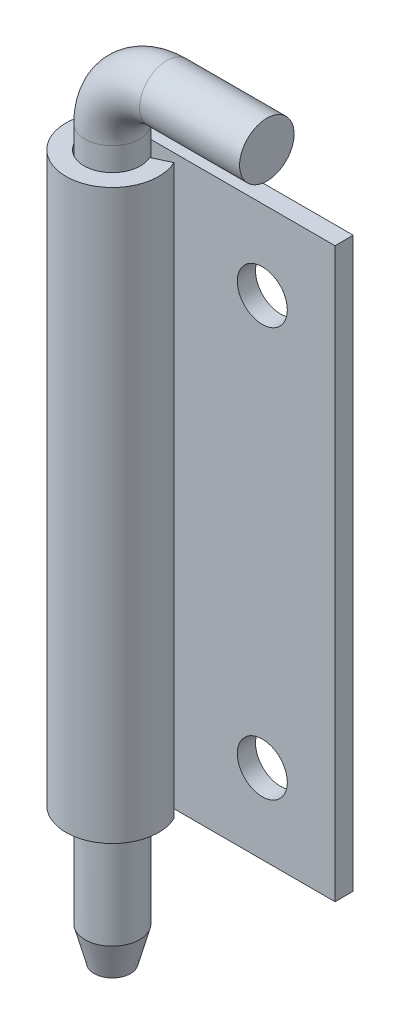
from build123d import *

# Parameters (mm, degrees)
SKETCH_2_R          = 3
EXTRUDE_1_DEPTH     = 62.5
SKETCH_5_R          = 2.75
CUT_EXTRUDE_2_DEPTH = 92.903210052
CHAMFER_1_SIZE      = 1
CHAMFER_1_SIZE2     = 3.732050808


with BuildPart() as part:
    # 扫描1: sweep along a path in 草图1
    with BuildLine(Plane.XY) as sweep_1_path:
        Line((0, 0), (0, 80))
        ThreePointArc((0, 80), (1.757359313, 84.242640687), (6, 86))
        Line((6, 86), (17, 86))
    # 草图2 → 扫描1 (sweep)
    with BuildSketch(Plane(origin=(0, 0, 0), x_dir=(1, 0, 0), z_dir=(0, 1, 0))):
        Circle(SKETCH_2_R)
    sweep(path=sweep_1_path.line)

    # 倒角1
    chamfer_1_edges = [part.edges().sort_by_distance(p)[0] for p in [
        (-3, 0, 0),
    ]]
    chamfer_1_side = [part.faces().sort_by_distance(p)[0] for p in [
        (0, 0, 0),
    ]]
    chamfer(chamfer_1_edges, length=CHAMFER_1_SIZE, length2=CHAMFER_1_SIZE2, reference=chamfer_1_side[0])


with BuildPart() as body_2:
    # 草图3 → 凸台-拉伸1 (new body)
    with BuildSketch(Plane(origin=(0, 15, 0), x_dir=(-1, 0, 0), z_dir=(0, -1, 0))):
        with BuildLine():
            Line((0, 3.1), (-21.4, 3.1))
            Line((-21.4, 3.1), (-21.4, 5.1))
            Line((-21.4, 5.1), (0, 5.1))
            ThreePointArc((0, 5.1), (2.740228003, -4.301296374), (-4.622169714, 2.155353135))
            Line((-4.622169714, 2.155353135), (-2.80955414, 1.310116611))
            ThreePointArc((-2.80955414, 1.310116611), (1.665628786, -2.614513482), (0, 3.1))
        make_face()
    extrude(amount=-EXTRUDE_1_DEPTH)

    # 草图5 → 切除-拉伸2 (cut, through all)
    with BuildSketch(Plane.XY.offset(-3.1)):
        with Locations((13.4, 23.75)):
            Circle(SKETCH_5_R)
        with Locations((13.4, 68.75)):
            Circle(SKETCH_5_R)
    extrude(amount=-CUT_EXTRUDE_2_DEPTH, mode=Mode.SUBTRACT)


solid = Compound([part.part, body_2.part])
